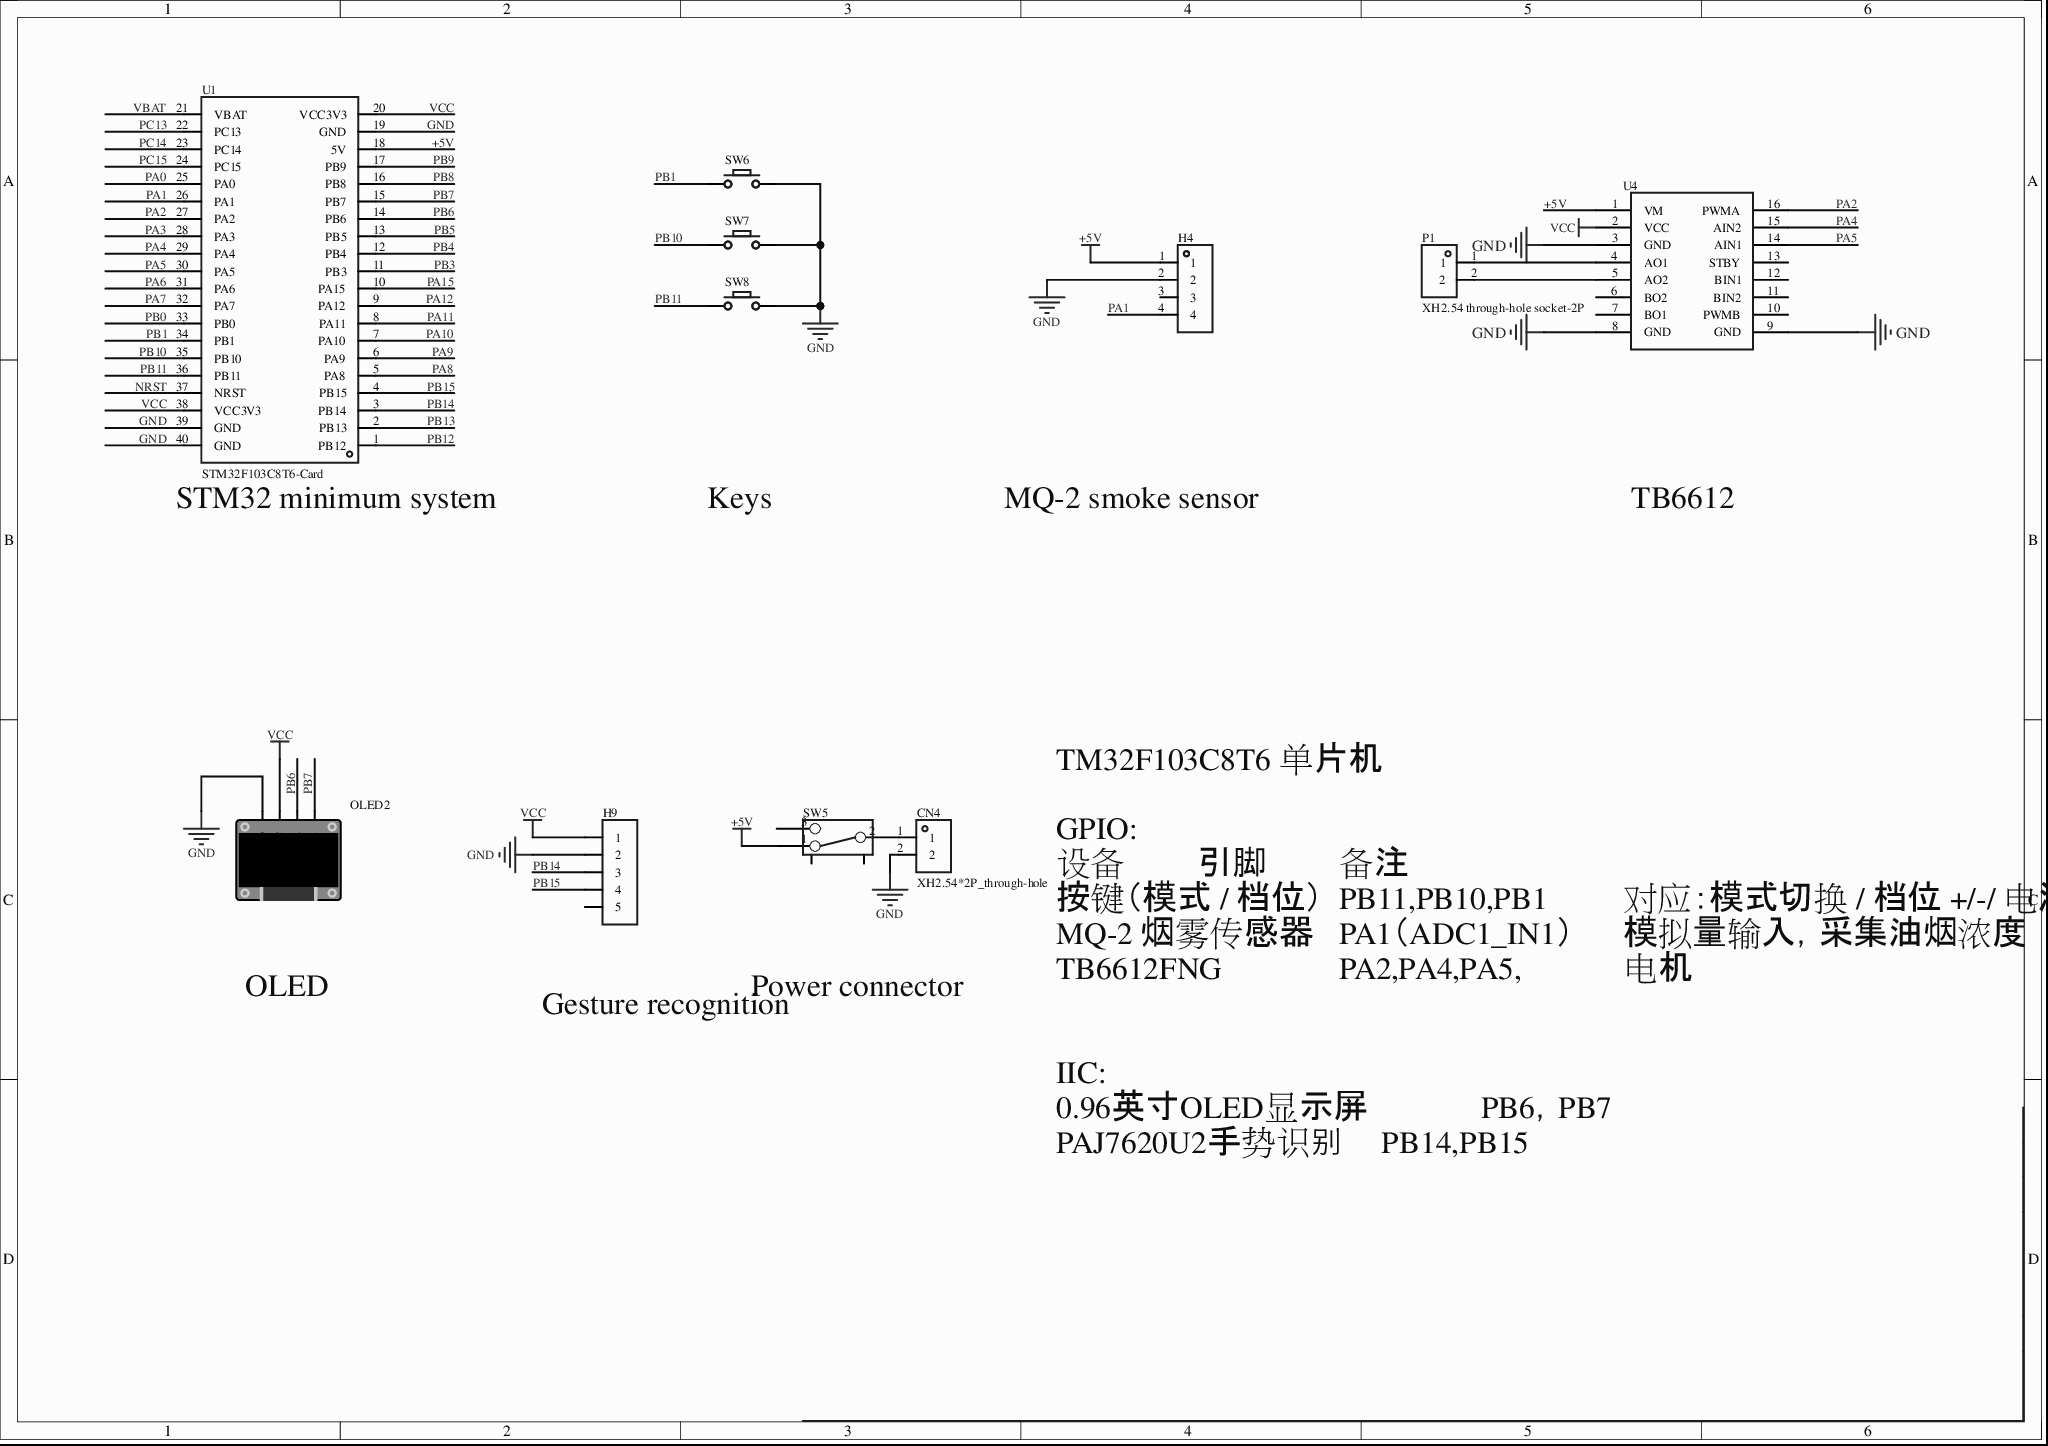
[diagram p0: MISC89068-3.schdoc]
# Altium project MISC89068-2.PrjPcb
1 sheet, 11 parts. Net scope: global (net labels, ports and power ports of the same name join across sheets).
Board file: MISC89068.pcbdoc

## Sheet MISC89068-3.schdoc
size 297 x 209 mm; Version: V1.0; @Project Name: MISC89068; @Page Count: 1; @Update Date: 2026-05-03; @Create Date: 2026-05-03; @Schematic Name: MISC89068; @Page No: 1; @Create Time: 23:22:16; @Update Time: 17:32:40; @Board Name: MISC89068

### Parts
CN4  XH2.54*2P_through-hole  [CONN-TH_2P-P2.50-XH2.54-2P]
H4  (no value)  [HDR-TH_4P-P2.54-V-F]
H9  (no value)  [HDR-TH_5P-P2.54-V-F]
OLED2  (no value)  [0.96OLED_4P]
P1  XH2.54 through-hole socket-2P  [CONN-TH_XH2.54-2P]
SW5  (no value)  [拨动开关]
SW6  (no value)  [Key_TH_3.5x6x4.3]
SW7  (no value)  [Key_TH_3.5x6x4.3]
SW8  (no value)  [Key_TH_3.5x6x4.3]
U1  STM32F103C8T6-Card  [CONN-TH_L53.3-W22.9_STM32F103C8T6-CARD]
U4  (no value)  [tb6612]

### Nets
+5V: H4.1 SW5.1 U1.18(5V) U4.1(VM)
GND: CN4.2 H4.2 H9.2 OLED2.1(GND) SW6.B SW7.B SW8.B U1.19(GND) U1.39(GND) U1.40(GND) U4.3(GND) U4.8(GND) U4.9(GND)
VCC: H9.1 OLED2.2(VCC) U1.20(VCC3V3) U1.38(VCC3V3) U4.2(VCC)
NRST: U1.37(NRST)
PA0: U1.25(PA0)
PA1: H4.4 U1.26(PA1)
PA2: U1.27(PA2) U4.16(PWMA)
PA3: U1.28(PA3)
PA4: U1.29(PA4) U4.15(AIN2)
PA5: U1.30(PA5) U4.14(AIN1)
PA6: U1.31(PA6)
PA7: U1.32(PA7)
PA8: U1.5(PA8)
PA9: U1.6(PA9)
PA10: U1.7(PA10)
PA11: U1.8(PA11)
PA12: U1.9(PA12)
PA15: U1.10(PA15)
PB0: U1.33(PB0)
PB1: SW6.A U1.34(PB1)
PB3: U1.11(PB3)
PB4: U1.12(PB4)
PB5: U1.13(PB5)
PB6: OLED2.3(SCL) U1.14(PB6)
PB7: OLED2.4(SDA) U1.15(PB7)
PB8: U1.16(PB8)
PB9: U1.17(PB9)
PB10: SW7.A U1.35(PB10)
PB11: SW8.A U1.36(PB11)
PB12: U1.1(PB12)
PB13: U1.2(PB13)
PB14: H9.3 U1.3(PB14)
PB15: H9.4 U1.4(PB15)
PC13: U1.22(PC13)
PC14: U1.23(PC14)
PC15: U1.24(PC15)
VBAT: U1.21(VBAT)
NetCN4_1: CN4.1 SW5.2
NetP1_1: P1.1 U4.4(AO1)
NetP1_2: P1.2 U4.5(AO2)

Not connected (* = marked no-connect by the designer): H4 3; H9 5; SW5 3 4 5; U4 6(BO2) 7(BO1) 10(PWMB) 11(BIN2) 12(BIN1) 13(STBY)

### Notes on the sheet
- (near U1) STM32 minimum system
- Keys
- MQ-2 smoke sensor
- TB6612
- TM32F103C8T6 单片机
  GPIO:
  设备	引脚	备注
  按键（模式 / 档位）	PB11,PB10,PB1	对应：模式切换 / 档位 +/-/ 电源
  MQ-2 烟雾传感器	PA1（ADC1_IN1）	模拟量输入，采集油烟浓度
  TB6612FNG 	PA2,PA4,PA5,	电机
  IIC:
  0.96英寸OLED显示屏	PB6，PB7
  PAJ7620U2手势识别     PB14,PB15
- OLED
- Gesture recognition
- Power connector

### Library data of the parts
CN4 = XH2.54*2P_直插: 3D Model: 325c595e30db4df8abe76612dd40b0fa0819f05c4eef4c71ace90d822a990e87; 3D Model Transform: 295.275,228.346,0,180,0,0,-0.002,-20.079,-137.795; AddInBom: yes; Device: XH2.54*2P_through-hole; Symbol: XH2.54*2P_through-hole; LCSC Part Name: XH2.54*2P_直插; Supplier Part: C9900008615; Manufacturer Part: XH2.54*2P_直插; Supplier Footprint: XH2.54_2P; JLCPCB Part Class: Extended Part; Supplier: LCSC; FootprintName: CONN-TH_2P-P2.50-XH2.54-2P; ConvertToPcb: yes; ModelName: CONN-TH_2P-P2.50-XH2.54-2P
H4 = HDR-F_2.54_1x4P: Symbol: 2.54-1*4P female; ConvertToPcb: yes; ModelId: d187812051054f85879fcaa51a310d8e0819f05c4eef4c71ace90d822a990e87; ModelTransform: 419.6842,98.464,0,0,0,0,0,0,-118.11; Device: HDR-F_2.54_1x4P; FootprintName: HDR-TH_4P-P2.54-V-F; AddInBom: yes; SupplierPart: C2718488; Supplier Footprint: 插件; ModelName: HDR-TH_4P-P2.54-V-F
H9 = HDR-F_2.54_1x5P: Symbol: Header-Female-2.54_1x5; 3D Model: f49cb6116a3d45e5a64915bf3e00773f; 3D Model Transform: 519.684,98.464,0,0,0,0,0,0,-124.016; ConvertToPcb: yes; Device: HDR-F_2.54_1x5P; Supplier Part: C50950; Supplier Footprint: 插件; AddInBom: yes; FootprintName: HDR-TH_5P-P2.54-V-F; ModelName: HDR-TH_5P-P2.54-V-F
OLED2 = 0.96OLED模块_4P: Symbol: 0.96OLED module_4P; 3D Model: 79c000fdb68d45a296c2e9bedf4f9055; 3D Model Transform: 1393.69792,1318.895,0,0,0,0,0,-560.079,-137.795; ConvertToPcb: yes; Device: 0.96OLED module_4P; Supplier Footprint: 插件; AddInBom: yes; FootprintName: 0.96OLED_4P; ModelName: 0.96OLED_4P
P1 = XH2.54直插座-2P: AddInBom: yes; ModelId: c3cc11bd8b8748c1ae6bc231aac3a1ff0819f05c4eef4c71ace90d822a990e87; ModelTransform: 296.889,230.315,0,0,0,0,0,26.653,-137.795; Symbol: XH2.54 through-hole socket-2P; Device: XH2.54 through-hole socket-2P; LCSC Part Name: XH2.54直插座-2P; SupplierPart: C9900016957; ManufacturerPart: XH2.54直插座-2P; Supplier Footprint: XH2.54-2; JLCPCB Part Class: Extended Part; Supplier: LCSC; ConvertToPcb: yes; FootprintName: CONN-TH_XH2.54-2P; ModelName: CONN-TH_XH2.54-2P
SW5 = 拨动开关_正: Device: Toggle switch_upright; Symbol: Toggle switch; ConvertToPcb: yes; ModelId: 4321fe59a4074cbfb4989553f297c68f0819f05c4eef4c71ace90d822a990e87; ModelName: SW-TH_SS-12D02-VG4; ModelTransform: 370.09,208.7,472.35,0,0,0,0,0,-110; FootprintName: Toggle switch; AddInBom: yes; Supplier Footprint: 插件
SW6-SW8 = Key_TH_3.5x6x4.3: ConvertToPcb: yes; ModelId: c3523f9014d949d7ba5445190a3178990819f05c4eef4c71ace90d822a990e87; ModelName: SW-TH_L6.0-W3.5-H5.0-P6.5; ModelTransform: 308.49,137.8,335.08,0,0,0,0,0,-129.92; Symbol: Key_TH_3.5x6x4.3; Device: Key_TH_3.5x6x4.3; AddInBom: yes; Supplier Footprint: 插件; FootprintName: Key_TH_3.5x6x4.3
U1 = STM32F103C8T6-Card: AddInBom: yes; Device: STM32F103C8T6-Card; Symbol: STM32F103C8T6-CARD; FootprintName: CONN-TH_L53.3-W22.9_STM32F103C8T6-CARD; LCSC Part Name: STM32F103C8T6-Card; SupplierPart: C9900077949; ManufacturerPart: STM32F103C8T6-Card; Supplier Footprint: 插件; Supplier: LCSC; ConvertToPcb: yes
U4 = tb6612: AddInBom: yes; Symbol: tb6612; Device: tb6612; JLCPCB Part Class: Extended library; ConvertToPcb: yes; FootprintName: tb6612